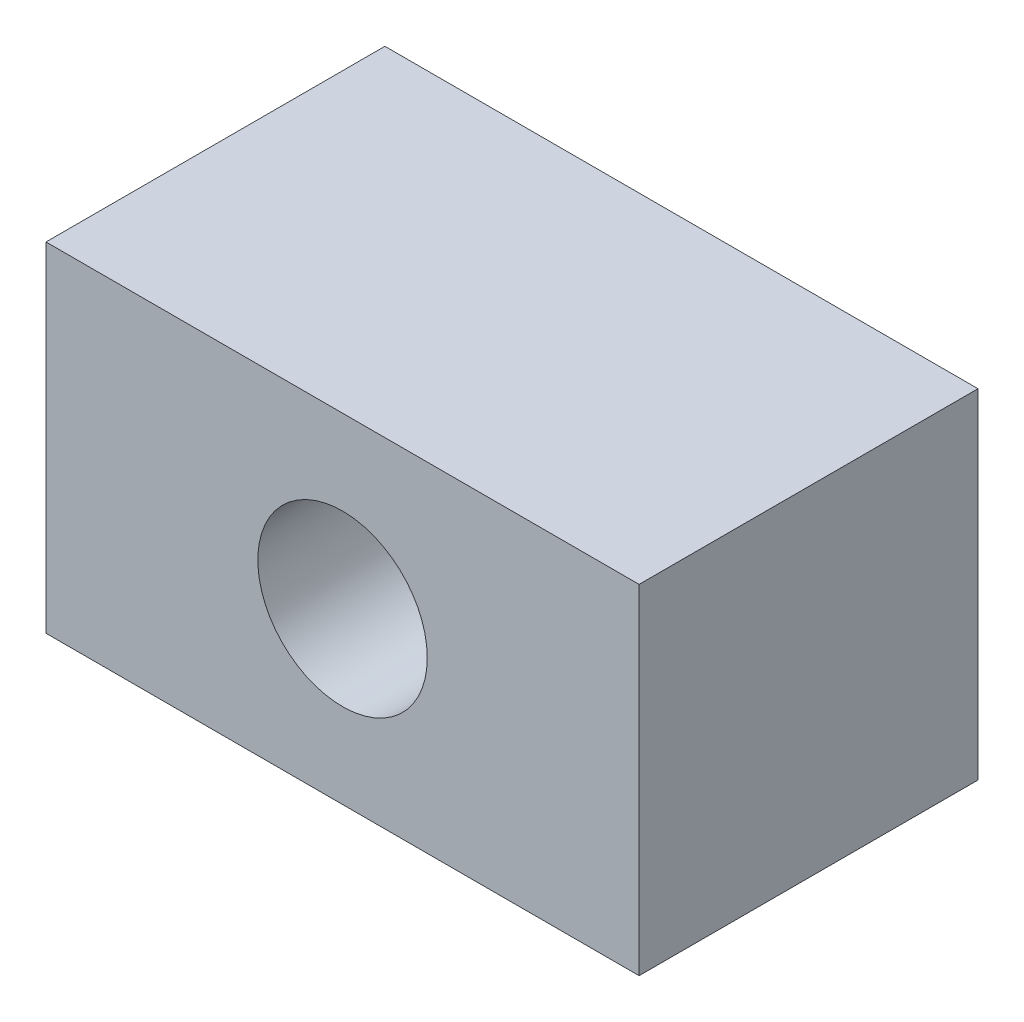
from build123d import *

# Parameters (mm, degrees)
SKETCH1_W           = 35
SKETCH1_H           = 20
SKETCH1_R           = 5
BOSS_EXTRUDE1_DEPTH = 20


with BuildPart() as part:
    # Sketch1 → Boss-Extrude1 (new body)
    with BuildSketch(Plane.XY):
        Rectangle(SKETCH1_W, SKETCH1_H)
        Circle(SKETCH1_R, mode=Mode.SUBTRACT)
    extrude(amount=BOSS_EXTRUDE1_DEPTH)


solid = part.part
